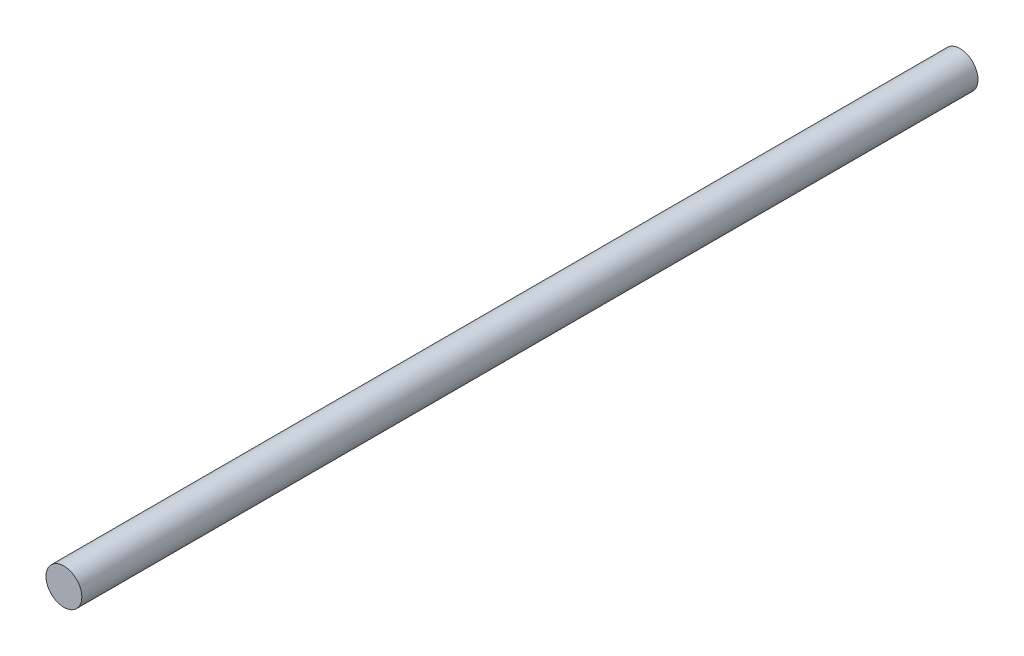
SolidWorks part; units mm, degrees
ref_plane "Front Plane" through (0, 0, 0) normal (0, 0, 1) x (1, 0, 0)
ref_plane "Top Plane" through (0, 0, 0) normal (0, 1, 0) x (1, 0, 0)
ref_plane "Right Plane" through (0, 0, 0) normal (1, 0, 0) x (0, 0, -1)
other "Configuration Table"
sketch "Sketch1" plane through (0, 0, 0) normal (0, 0, 1) x (1, 0, 0)
  circle A0 centre (0, 0) radius 5
  dimension "D1" = 10
extrude "Boss-Extrude1" add sketch "Sketch1" along normal blind 250
